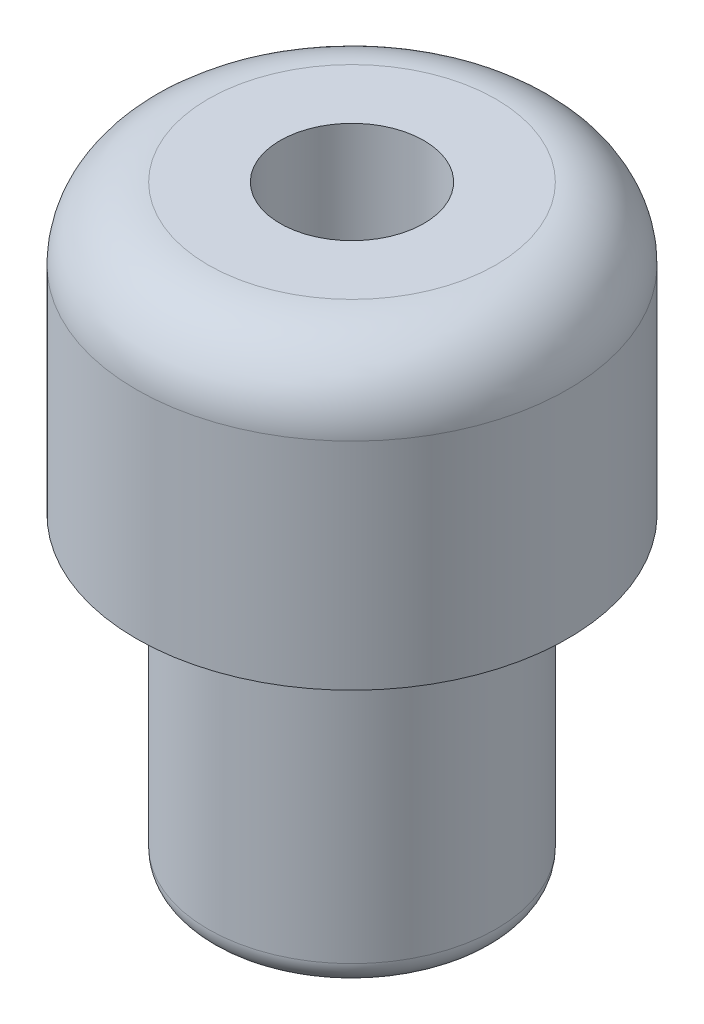
from build123d import *

# Parameters (mm, degrees)
FILLET_1_R = 3
FILLET_2_R = 1


with BuildPart() as part:
    # 草图1 → 旋转1 (revolve)
    with BuildSketch(Plane.XY, mode=Mode.PRIVATE) as revolve_1_sk:
        Polygon((3, 25), (3, 0), (6, 0), (6, 13), (9, 13), (9, 25), align=None)
    revolve(revolve_1_sk.sketch.rotate(Axis((0, 0, 0), (0, 1, 0)), 90), axis=Axis((0, 0, 0), (0, 1, 0)))

    # 圆角1
    fillet_1_edges = [part.edges().sort_by_distance(p)[0] for p in [
        (0, 25, 9),
    ]]
    fillet(fillet_1_edges, radius=FILLET_1_R)

    # 圆角2
    fillet_2_edges = [part.edges().sort_by_distance(p)[0] for p in [
        (0, 0, 6),
    ]]
    fillet(fillet_2_edges, radius=FILLET_2_R)


solid = part.part
